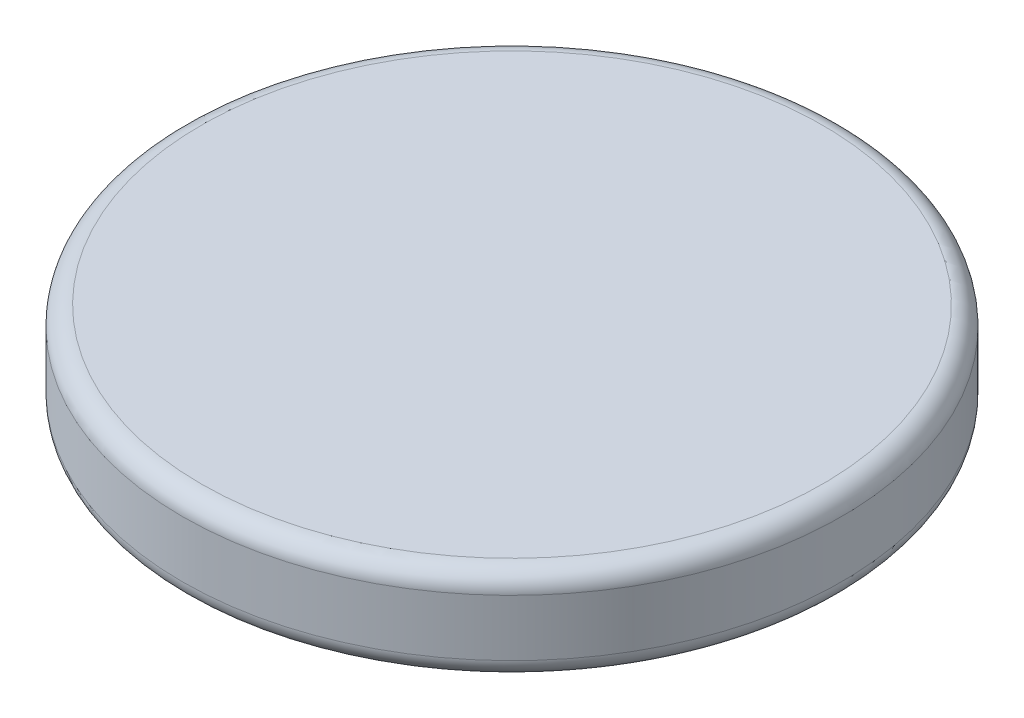
from build123d import *

# Parameters (mm, degrees)
SKETCH_1_R      = 17.5
EXTRUDE_1_DEPTH = 2.5
FILLET_1_R      = 1


with BuildPart() as part:
    # 草图1 → 凸台-拉伸1 (new, symmetric)
    with BuildSketch(Plane(origin=(0, 0, 0), x_dir=(1, 0, 0), z_dir=(0, 1, 0))):
        with Locations(Location((0, 0, 0), (0, 0, 270))):
            Circle(SKETCH_1_R)
    extrude(amount=EXTRUDE_1_DEPTH, both=True)

    # 圆角1
    fillet_1_edges = [part.edges().sort_by_distance(p)[0] for p in [
        (0, -2.5, -17.5),
        (0, 2.5, -17.5),
    ]]
    fillet(fillet_1_edges, radius=FILLET_1_R)


solid = part.part
